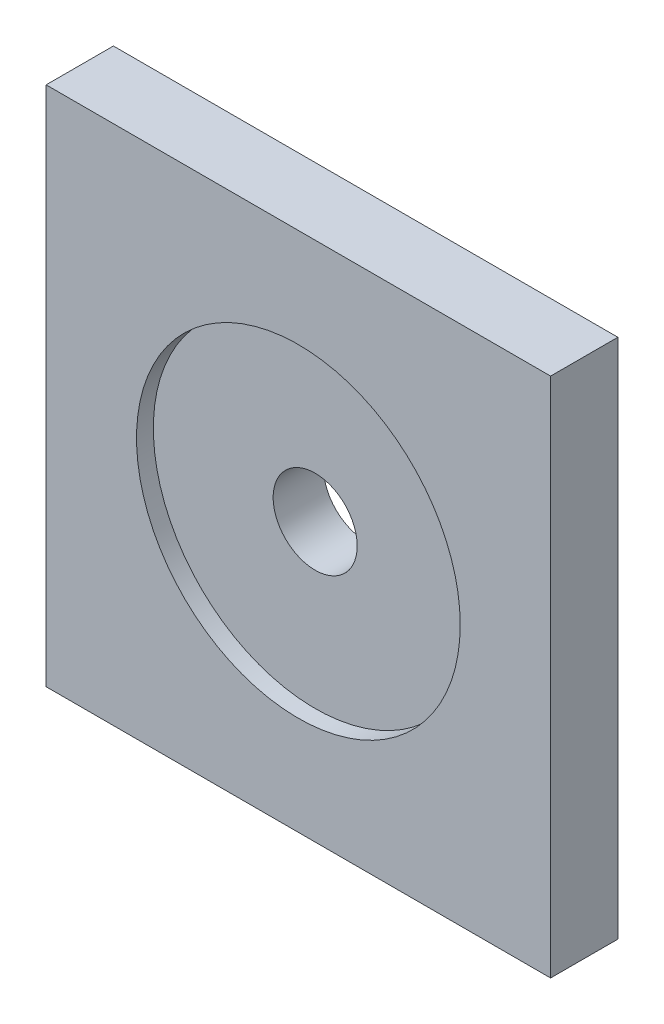
from build123d import *

# Parameters (mm, degrees)
SKETCH1_W           = 60
SKETCH1_H           = 62
BOSS_EXTRUDE1_DEPTH = 8
SKETCH3_R           = 19.25
CUT_EXTRUDE1_DEPTH  = 2
SKETCH4_R           = 5
CUT_EXTRUDE2_DEPTH  = 44.554563481


with BuildPart() as part:
    # Sketch1 → Boss-Extrude1 (new body)
    with BuildSketch(Plane.XY):
        Rectangle(SKETCH1_W, SKETCH1_H)
    extrude(amount=BOSS_EXTRUDE1_DEPTH)

    # Sketch3 → Cut-Extrude1 (cut)
    with BuildSketch(Plane.XY.offset(8)):
        Circle(SKETCH3_R)
    extrude(amount=-CUT_EXTRUDE1_DEPTH, mode=Mode.SUBTRACT)

    # Sketch4 → Cut-Extrude2 (cut, through all)
    with BuildSketch(Plane.XY.offset(6)):
        Circle(SKETCH4_R)
    extrude(amount=-CUT_EXTRUDE2_DEPTH, mode=Mode.SUBTRACT)


solid = part.part
